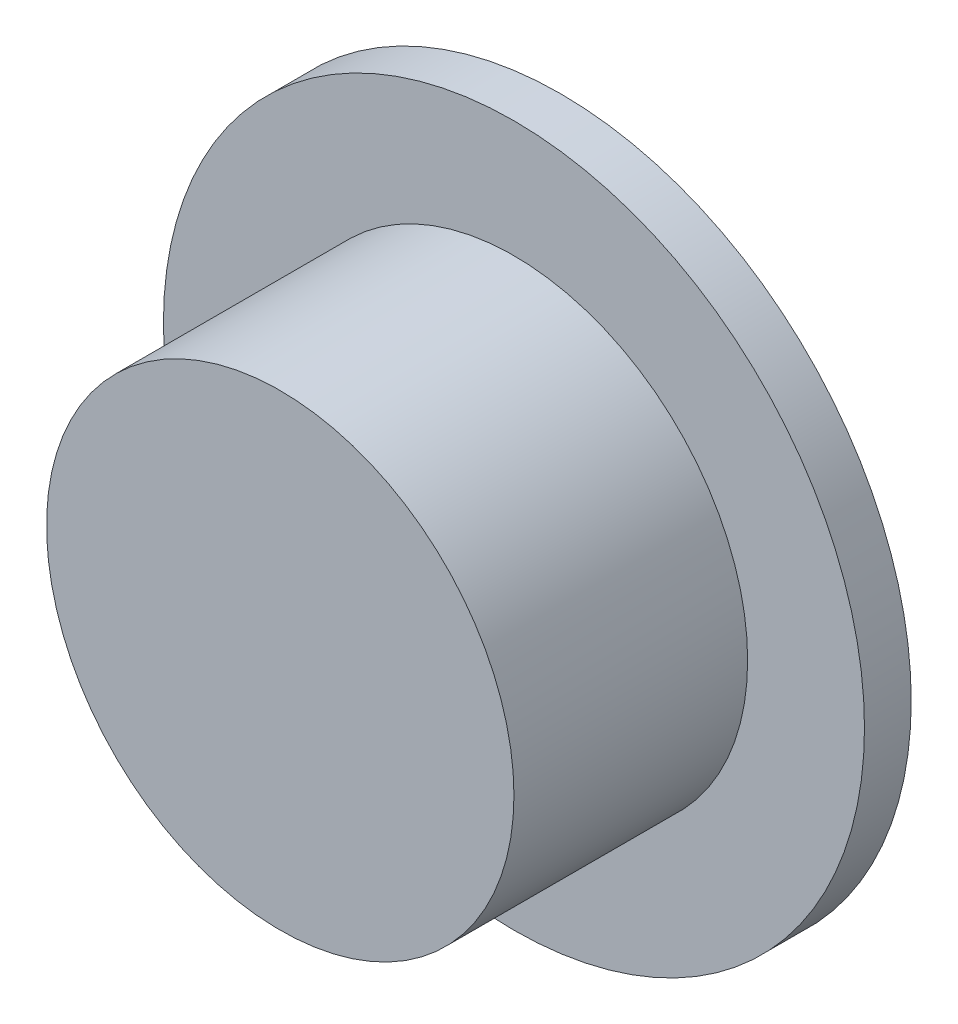
SolidWorks part; units mm, degrees
ref_plane "Front Plane" through (0, 0, 0) normal (0, 0, 1) x (1, 0, 0)
ref_plane "Top Plane" through (0, 0, 0) normal (0, 1, 0) x (1, 0, 0)
ref_plane "Right Plane" through (0, 0, 0) normal (1, 0, 0) x (0, 0, -1)
other "Configuration Table"
sketch "Sketch1" plane through (0, 0, 0) normal (0, 0, 1) x (1, 0, 0)
  circle A0 centre (0, 0) radius 15
  dimension "D1" = 30
extrude "Boss-Extrude1" add sketch "Sketch1" along normal blind 2
sketch "Sketch2" plane through (0, 0, 2) normal (0, 0, 1) x (1, 0, 0)
  circle A0 centre (0, 0) radius 10
  dimension "D1" = 20
extrude "Boss-Extrude2" add sketch "Sketch2" along normal blind 10
